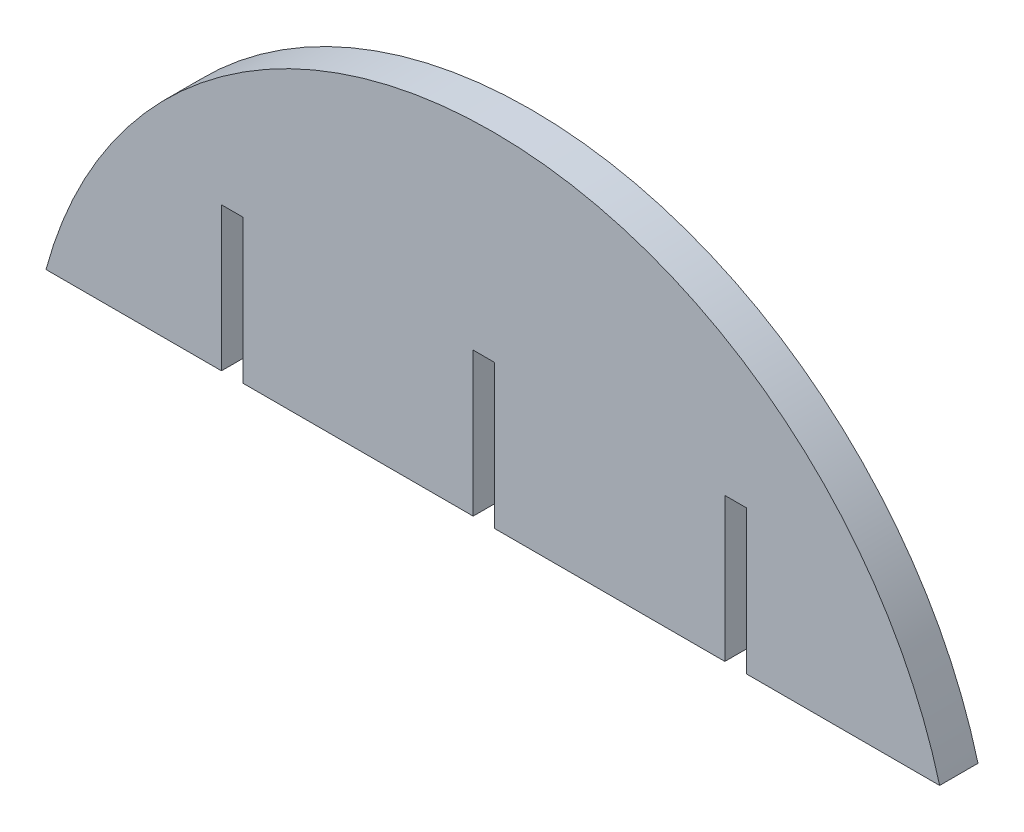
SolidWorks part; units mm, degrees
material "Q235B"
ref_plane "Front Plane" through (0, 0, 0) normal (0, 0, 1) x (1, 0, 0)
ref_plane "Top Plane" through (0, 0, 0) normal (0, 1, 0) x (1, 0, 0)
ref_plane "Right Plane" through (0, 0, 0) normal (1, 0, 0) x (0, 0, -1)
sketch "Sketch1" plane through (0, 0, 0) normal (0, 0, 1) x (1, 0, 0)
  line L0 (-94.65, 0) -> (98.35, 0)
  arc A0 (98.35, 0) -> (-94.65, 0) centre (1.85, 0) ccw
  dimension "D1" = 96.5
extrude "Boss-Extrude1" add sketch "Sketch1" along normal blind 8
sketch "Sketch2" plane through (0, 0, 8) normal (0, 0, 1) x (1, 0, 0)
  line L0 (-94.65, 0) -> (-94.65, 25)
  line L1 (-94.65, 25) -> (109.4523, 25)
  line L2 (109.4523, 25) -> (98.6492, -24.1744)
  line L3 (98.6492, -24.1744) -> (-94.65, 0)
extrude "Cut-Extrude1" cut sketch "Sketch2" against normal blind 10
sketch "Sketch3" plane through (0, 0, 0) normal (0, 0, -1) x (-1, 0, 0)
  line L0 (-95.0554, 25) -> (91.3554, 25) construction
  line L1 (-2.25, 55) -> (2.25, 55)
  line L2 (-2.25, 25) -> (2.25, 25)
  line L3 (54.75, 25) -> (50.25, 25)
  line L4 (2.25, 25) -> (2.25, 55)
  line L5 (-50.25, 25) -> (-54.75, 25)
  line L6 (-50.25, 25) -> (-50.25, 55)
  line L7 (-50.25, 55) -> (-54.75, 55)
  line L8 (-54.75, 25) -> (-54.75, 55)
  line L9 (-2.25, 55) -> (-2.25, 25)
  line L10 (50.25, 25) -> (50.25, 55)
  line L11 (54.75, 25) -> (54.75, 55)
  line L12 (54.75, 55) -> (50.25, 55)
  dimension "D1" = 30
  dimension "D2" = 48
  dimension "D3" = 4.5
  dimension "D4" = 2.25
  dimension "D5" = 4.5
  dimension "D6" = 30
  dimension "D7" = 48
extrude "Cut-Extrude2" cut sketch "Sketch3" against normal blind 10
